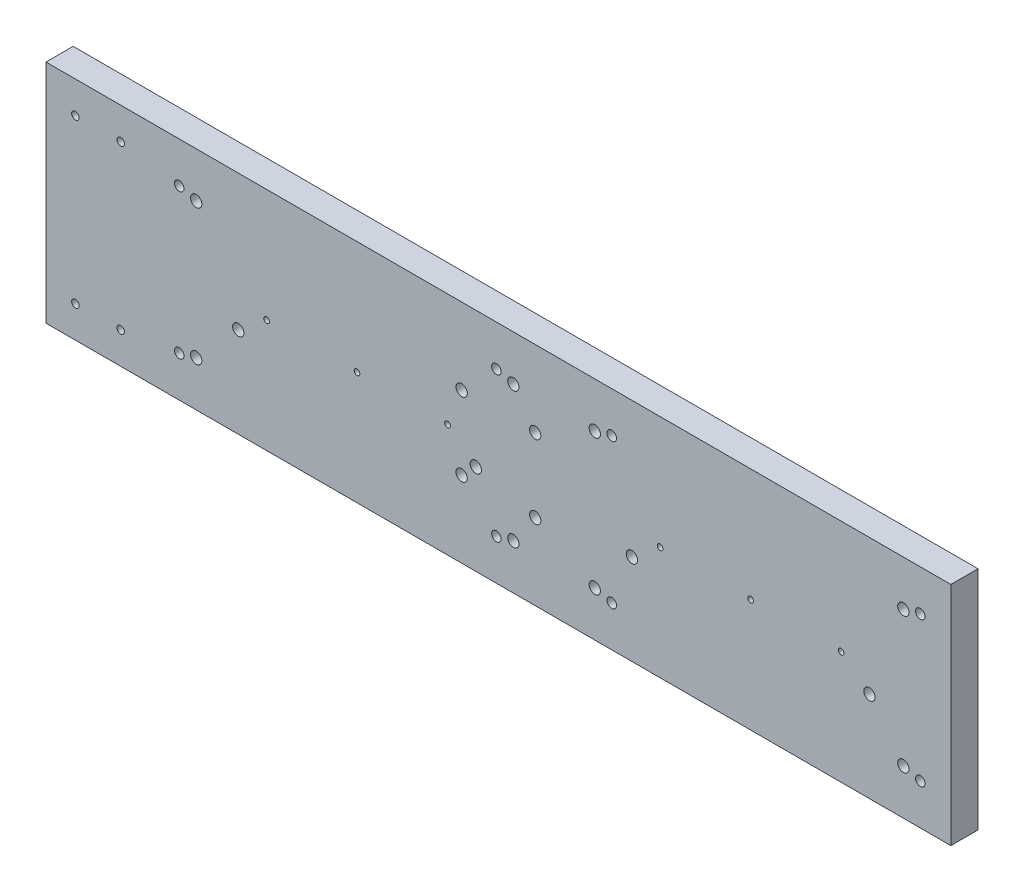
SolidWorks part; units mm, degrees
ref_plane "Front" through (0, 0, 0) normal (0, 0, 1) x (1, 0, 0)
ref_plane "Top" through (0, 0, 0) normal (0, 1, 0) x (1, 0, 0)
ref_plane "Right" through (0, 0, 0) normal (1, 0, 0) x (0, 0, -1)
sketch "Sketch1" plane through (0, 0, 0) normal (0, 0, 1) x (1, 0, 0)
  line L1 (0, 0) -> (400, 0)
  line L2 (0, 0) -> (0, 100)
  line L3 (0, 100) -> (400, 100)
  line L4 (400, 0) -> (400, 100)
  dimension "D1" = 400
  dimension "D2" = 100
extrude "Boss-Extrude1" add sketch "Sketch1" along normal blind 12
hole_wizard "M4 Tapped Hole1" positions "Sketch3" profile "Sketch2" tap size "M4" standard "ISO" end condition through all
sketch "Sketch3" plane through (0, 0, 12) normal (0, 0, 1) x (1, 0, 0)
  line L0 (0, 0) -> (400, 0) construction
  line L1 (0, 100) -> (0, 0) construction
  point P0 (13, 14)
  point P1 (13, 86)
  point P3 (33, 86)
  point P5 (33, 14)
  dimension "D1" = 14
  dimension "D2" = 72
  dimension "D3" = 13
  dimension "D4" = 20
sketch "Sketch2" plane through (13, 14, 12) normal (1, 0, 0) x (0, -1, 0)
  line L0 (0, 0) -> (0, 12)
  line L1 (0, 12) -> (1.65, 12)
  line L2 (1.65, 12) -> (1.65, 0)
  line L5 (1.65, 0) -> (0, 0)
  line L11 (0, -6.35) -> (0, 107.95) construction
  dimension "Thru Tap Drill Dia." = 3.3
  dimension "Thru Tap Drill Depth" = 12
cosmetic thread "Hole Thread1" parameters "D2"=4
cosmetic thread "Hole Thread2" parameters "D2"=4
cosmetic thread "Hole Thread3" parameters "D2"=4
cosmetic thread "Hole Thread4" parameters "D2"=4
hole_wizard "M5 Tapped Hole1" positions "Sketch5" profile "Sketch4" tap size "M5" standard "ISO" end condition through all
sketch "Sketch5" plane through (0, 0, 12) normal (0, 0, 1) x (1, 0, 0)
  line L0 (0, 0) -> (400, 0) construction
  line L2 (0, 100) -> (0, 0) construction
  point P0 (58.9, 82)
  point P1 (58.9, 18)
  point P11 (199.1, 82)
  point P13 (199.1, 18)
  point P15 (250.1, 18)
  point P17 (250.1, 82)
  point P19 (386.5, 82)
  point P21 (386.5, 18)
  dimension "D1" = 64
  dimension "D2" = 18
  dimension "D3" = 58.9
  dimension "D4" = 140.2
  dimension "D5" = 51
  dimension "D6" = 136.4
sketch "Sketch4" plane through (58.9, 82, 12) normal (1, 0, 0) x (0, -1, 0)
  line L0 (0, 0) -> (0, 12)
  line L1 (0, 12) -> (2.1, 12)
  line L2 (2.1, 12) -> (2.1, 0)
  line L5 (2.1, 0) -> (0, 0)
  line L11 (0, -6.35) -> (0, 107.95) construction
  dimension "Thru Tap Drill Dia." = 4.2
  dimension "Thru Tap Drill Depth" = 12
cosmetic thread "Hole Thread5" parameters "D2"=5
cosmetic thread "Hole Thread6" parameters "D2"=5
cosmetic thread "Hole Thread7" parameters "D2"=5
cosmetic thread "Hole Thread8" parameters "D2"=5
cosmetic thread "Hole Thread9" parameters "D2"=5
cosmetic thread "Hole Thread10" parameters "D2"=5
cosmetic thread "Hole Thread11" parameters "D2"=5
cosmetic thread "Hole Thread12" parameters "D2"=5
sketch "Sketch6" plane through (0, 0, 12) normal (0, 0, 1) x (1, 0, 0)
  line L0 (0, 0) -> (400, 0) construction
  line L1 (0, 100) -> (0, 0) construction
  circle A0 centre (66.4, 80) radius 2.5
  circle A1 centre (66.4, 20) radius 2.5
  circle A2 centre (206.6, 80) radius 2.5
  circle A3 centre (206.6, 20) radius 2.5
  circle A4 centre (242.6, 20) radius 2.5
  circle A5 centre (242.6, 80) radius 2.5
  circle A6 centre (379, 80) radius 2.5
  circle A7 centre (379, 20) radius 2.5
  circle A8 centre (85, 40) radius 2.5
  circle A9 centre (190, 40) radius 2.5
  circle A10 centre (259, 40) radius 2.5
  circle A11 centre (364, 40) radius 2.5
  dimension "D1" = 5
  dimension "D2" = 60
  dimension "D3" = 20
  dimension "D4" = 66.4
  dimension "D5" = 140.2
  dimension "D6" = 36
  dimension "D7" = 136.4
  dimension "D8" = 85
  dimension "D9" = 105
  dimension "D10" = 69
  dimension "D11" = 105
  dimension "D12" = 40
extrude "Cut-Extrude1" cut sketch "Sketch6" against normal through all
hole_wizard "M6 Tapped Hole1" positions "Sketch8" profile "Sketch7" tap size "M6" standard "ISO" end condition through all
sketch "Sketch8" plane through (0, 0, 12) normal (0, 0, 1) x (1, 0, 0)
  line L0 (0, 100) -> (0, 0) construction
  line L1 (0, 0) -> (400, 0) construction
  line L2 (216.2635, 66.2635) -> (200, 50) construction
  line L3 (200, 50) -> (216.2635, 33.7365) construction
  circle A0 centre (200, 50) radius 23 construction
  point P0 (183.7365, 66.2635)
  point P10 (216.2635, 66.2635)
  point P12 (216.2635, 33.7365)
  point P14 (183.7365, 33.7365)
  dimension "D1" = 46
  dimension "D2" = 200
  dimension "D3" = 50
sketch "Sketch7" plane through (183.7365, 66.2635, 12) normal (1, 0, 0) x (0, -1, 0)
  line L0 (0, 0) -> (0, 12)
  line L1 (0, 12) -> (2.5, 12)
  line L2 (2.5, 12) -> (2.5, 0)
  line L5 (2.5, 0) -> (0, 0)
  line L11 (0, -6.35) -> (0, 107.95) construction
  dimension "Thru Tap Drill Dia." = 5
  dimension "Thru Tap Drill Depth" = 12
cosmetic thread "Hole Thread13" parameters "D2"=6
cosmetic thread "Hole Thread14" parameters "D2"=6
cosmetic thread "Hole Thread15" parameters "D2"=6
cosmetic thread "Hole Thread16" parameters "D2"=6
hole_wizard "M3 Tapped Hole1" positions "Sketch10" profile "Sketch9" tap size "M3" standard "ISO" end condition through all
sketch "Sketch10" plane through (0, 0, 12) normal (0, 0, 1) x (1, 0, 0)
  line L0 (0, 0) -> (400, 0) construction
  line L1 (0, 100) -> (0, 0) construction
  point P0 (97.5, 50)
  point P1 (137.5, 50)
  point P3 (177.5, 50)
  point P5 (271.5, 50)
  point P7 (311.5, 50)
  point P9 (351.5, 50)
  dimension "D1" = 50
  dimension "D2" = 97.5
  dimension "D3" = 40
  dimension "D4" = 40
  dimension "D5" = 94
  dimension "D6" = 40
  dimension "D7" = 40
sketch "Sketch9" plane through (97.5, 50, 12) normal (1, 0, 0) x (0, -1, 0)
  line L0 (0, 0) -> (0, 12)
  line L1 (0, 12) -> (1.25, 12)
  line L2 (1.25, 12) -> (1.25, 0)
  line L5 (1.25, 0) -> (0, 0)
  line L11 (0, -6.35) -> (0, 107.95) construction
  dimension "Thru Tap Drill Dia." = 2.5
  dimension "Thru Tap Drill Depth" = 12
cosmetic thread "Hole Thread17" parameters "D2"=3
cosmetic thread "Hole Thread18" parameters "D2"=3
cosmetic thread "Hole Thread19" parameters "D2"=3
cosmetic thread "Hole Thread20" parameters "D2"=3
cosmetic thread "Hole Thread21" parameters "D2"=3
cosmetic thread "Hole Thread22" parameters "D2"=3
